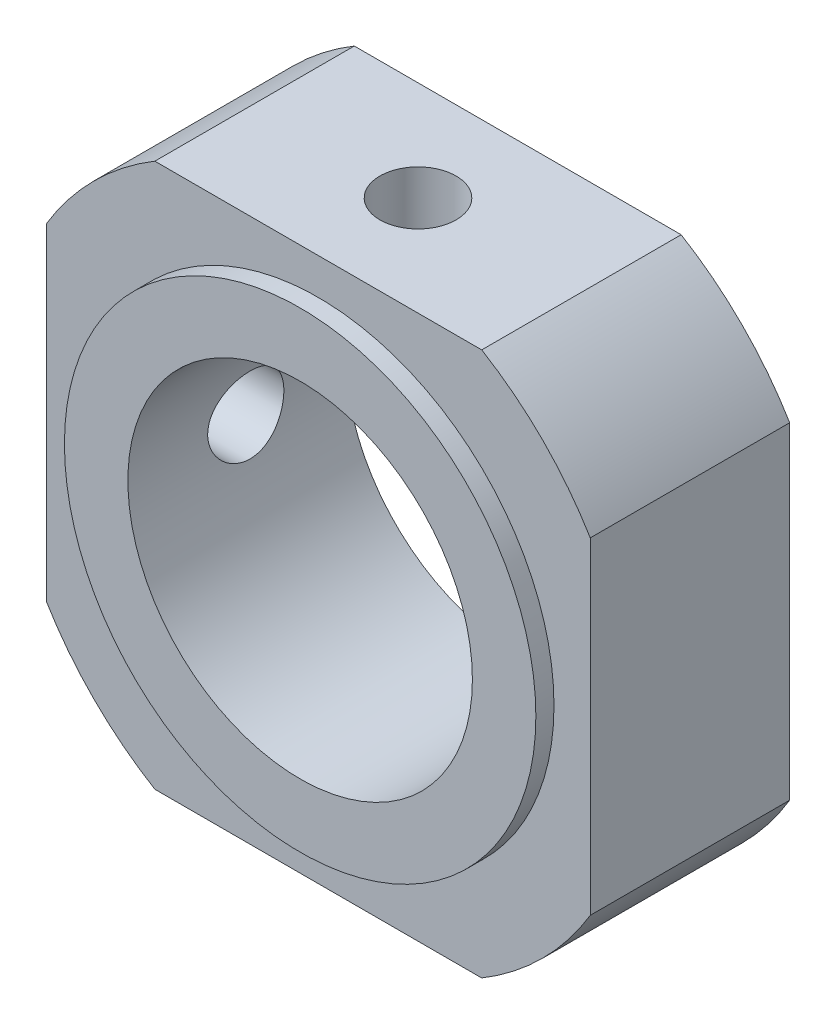
SolidWorks part; units mm, degrees
ref_plane "Front" through (0, 0, 0) normal (0, 0, 1) x (1, 0, 0)
ref_plane "Top" through (0, 0, 0) normal (0, 1, 0) x (1, 0, 0)
ref_plane "Right" through (0, 0, 0) normal (1, 0, 0) x (0, 0, -1)
sketch "Sketch1" plane through (0, 0, 0) normal (0, 0, 1) x (1, 0, 0)
  line L0 (-9.0139, 15) -> (9.0139, 15)
  line L1 (15, 9.0139) -> (15, -9.0139)
  line L2 (9.0139, -15) -> (-9.0139, -15)
  line L3 (-15, -9.0139) -> (-15, 9.0139)
  line L4 (0, 0) -> (0, 10.0983) construction
  line L5 (0, 0) -> (9.0373, 0) construction
  arc A0 (9.0139, -15) -> (15, -9.0139) centre (0, 0) ccw
  arc A1 (-15, -9.0139) -> (-9.0139, -15) centre (0, 0) ccw
  arc A2 (-9.0139, 15) -> (-15, 9.0139) centre (0, 0) ccw
  arc A3 (15, 9.0139) -> (9.0139, 15) centre (0, 0) ccw
  dimension "D1" = 35
  dimension "D2" = 30
  dimension "D3" = 30
extrude "Boss-Extrude1" add sketch "Sketch1" along normal blind 11
sketch "Sketch2" plane through (0, 0, 11) normal (0, 0, 1) x (1, 0, 0)
  circle A0 centre (0, 0) radius 13
  dimension "D1" = 26
extrude "Boss-Extrude2" add sketch "Sketch2" along normal blind 1
sketch "Sketch3" plane through (0, 0, 12) normal (0, 0, 1) x (1, 0, 0)
  circle A0 centre (0, 0) radius 9.5
  dimension "D1" = 19
extrude "Cut-Extrude1" cut sketch "Sketch3" against normal through all
cosmetic thread "Cosmetic Thread1" parameters "D2"=20
hole_wizard "M5 Tapped Hole1" positions "Sketch5" profile "Sketch4" tap size "M5" standard "GB"
sketch "Sketch5" plane through (-15, 0, 0) normal (-1, 0, 0) x (0, 0, 1)
  line L0 (0, 0) -> (11, 0) construction
  line L1 (11, -13) -> (11, 13) construction
  point P0 (5.5, 0)
sketch "Sketch4" plane through (-15, 0, 5.5) normal (0, 1, 0) x (0, 0, 1)
  line L0 (0, 0) -> (0, 5.5)
  line L1 (0, 5.5) -> (2.1, 5.5)
  line L2 (2.1, 5.5) -> (2.1, 0)
  line L5 (2.1, 0) -> (0, 0)
  line L11 (0, -6.35) -> (0, 107.95) construction
  dimension "通孔螺纹孔钻头直径" = 4.2
  dimension "通孔螺纹孔钻头深度" = 5.5
cosmetic thread "孔螺蚊线1" parameters "D2"=5
hole_wizard "M5 Tapped Hole2" positions "Sketch7" profile "Sketch6" tap size "M5" standard "GB"
sketch "Sketch7" plane through (0, 15, 0) normal (0, 1, 0) x (-1, 0, 0)
  line L0 (0, 0) -> (0, 12) construction
  line L1 (9.5, 12) -> (-9.5, 12) construction
  line L4 (-9.0139, 0) -> (9.0139, 0) construction
  point P0 (0, 5.5)
  dimension "D1" = 5.5
sketch "Sketch6" plane through (0, 15, 5.5) normal (1, 0, 0) x (0, 0, 1)
  line L0 (0, 0) -> (0, 5.5)
  line L1 (0, 5.5) -> (2.1, 5.5)
  line L2 (2.1, 5.5) -> (2.1, 0)
  line L5 (2.1, 0) -> (0, 0)
  line L11 (0, -6.35) -> (0, 107.95) construction
  dimension "通孔螺纹孔钻头直径" = 4.2
  dimension "通孔螺纹孔钻头深度" = 5.5
cosmetic thread "Cosmetic Thread2" parameters "D2"=5
